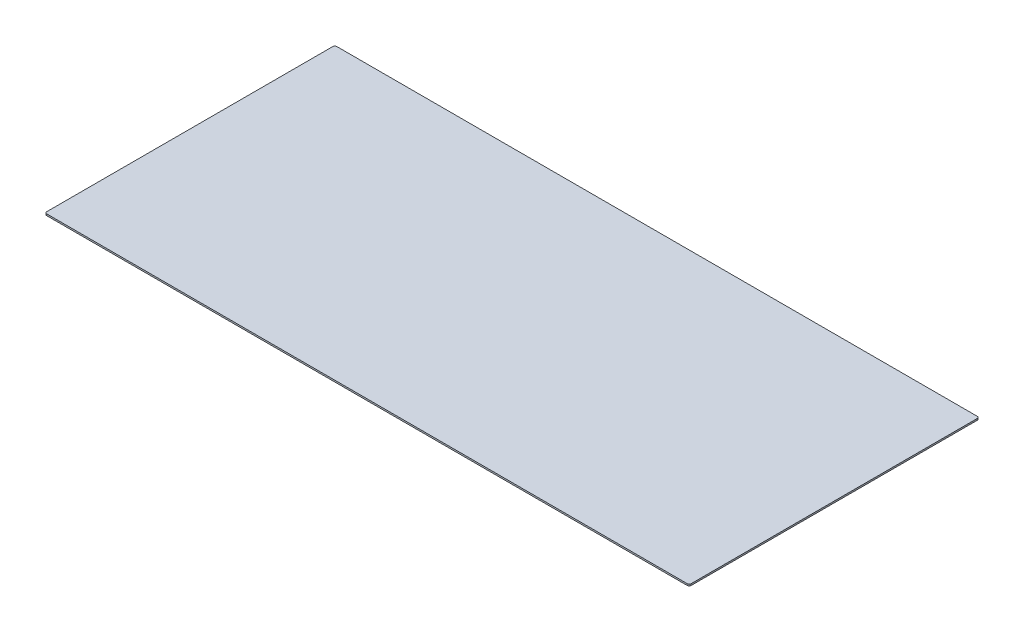
SolidWorks part; units mm, degrees
material "Q235"
ref_plane "Front Plane" through (0, 0, 0) normal (0, 0, 1) x (1, 0, 0)
ref_plane "Top Plane" through (0, 0, 0) normal (0, 1, 0) x (1, 0, 0)
ref_plane "Right Plane" through (0, 0, 0) normal (1, 0, 0) x (0, 0, -1)
sketch "Sketch1" plane through (0, 0, 0) normal (0, 1, 0) x (1, 0, 0)
  line L1 (-1000, 450) -> (1000, 450)
  line L2 (-1000, 450) -> (-1000, -450)
  line L3 (-1000, -450) -> (1000, -450)
  line L4 (1000, 450) -> (1000, -450)
  line L5 (-1000, 450) -> (1000, -450) construction
  line L6 (-1000, -450) -> (1000, 450) construction
  point P0 (0, 0)
  dimension "D1" = 2000
  dimension "D2" = 900
extrude "Boss-Extrude1" add sketch "Sketch1" along normal blind 5
fillet "Fillet1" radius 6 4 edges at (-1000, 2.5, 450) (1000, 2.5, 450) (1000, 2.5, -450) (-1000, 2.5, -450)
